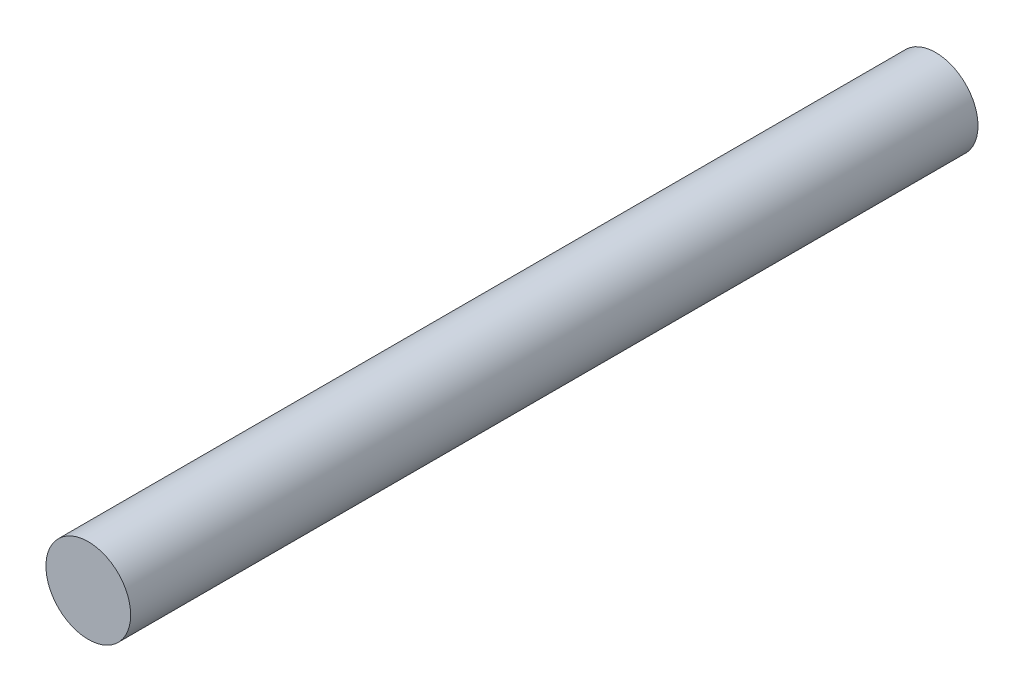
SolidWorks part; units mm, degrees
ref_plane "Front Plane" through (0, 0, 0) normal (0, 0, 1) x (1, 0, 0)
ref_plane "Top Plane" through (0, 0, 0) normal (0, 1, 0) x (1, 0, 0)
ref_plane "Right Plane" through (0, 0, 0) normal (1, 0, 0) x (0, 0, -1)
sketch "Sketch1" plane through (0, 0, 0) normal (0, 0, 1) x (1, 0, 0)
  circle A0 centre (0, 0) radius 2.5
  dimension "D1" = 5
extrude "Boss-Extrude1" add sketch "Sketch1" along normal blind 50
